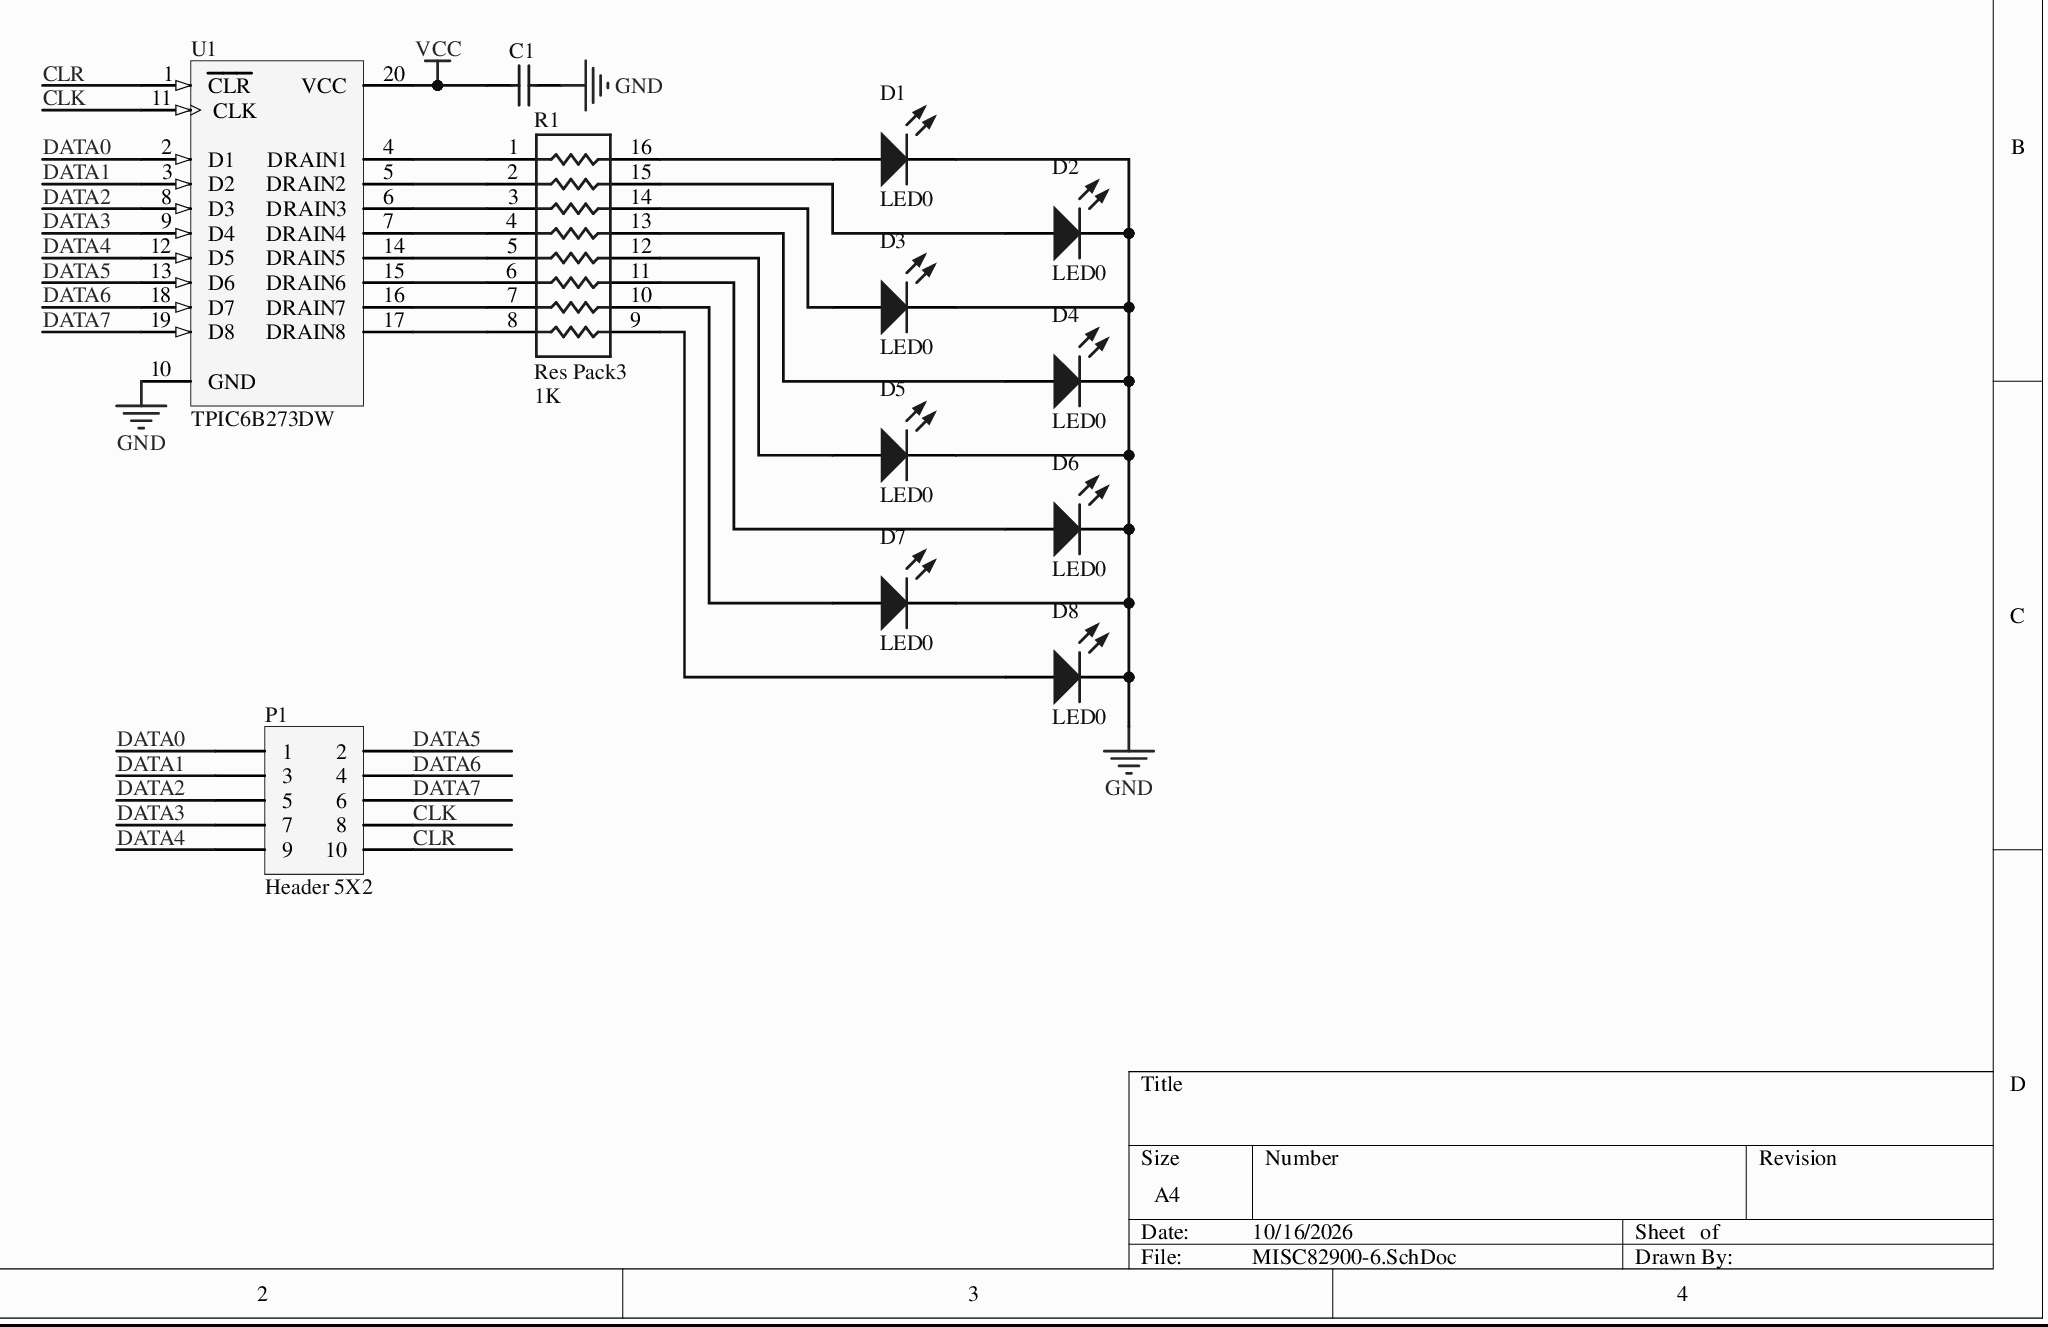
[diagram p0: MISC82900-6.SchDoc]
# Altium project MISC82900-2.PrjPcb
1 sheet, 12 parts. Net scope: global (net labels, ports and power ports of the same name join across sheets).
Board file: MISC82900.PcbDoc

## Sheet MISC82900-6.SchDoc
size A4

### Parts
C1  Cap  [RAD-0.3]  (value not drawn)
D1  LED0  [LED-0]
D2  LED0  [LED-0]
D3  LED0  [LED-0]
D4  LED0  [LED-0]
D5  LED0  [LED-0]
D6  LED0  [LED-0]
D7  LED0  [LED-0]
D8  LED0  [LED-0]
P1  Header 5X2  [HDR2X5]
R1  Res Pack3  value 1K  [SO-16_N]
U1  TPIC6B273DW  [DW020]

### Nets
GND: C1.2 D1.2(K) D2.2(K) D3.2(K) D4.2(K) D5.2(K) D6.2(K) D7.2(K) D8.2(K) U1.10(GND)
VCC: C1.1 U1.20(VCC)
CLK: P1.8 U1.11(CLK)
CLR: P1.10 U1.1(~{CLR})
DATA0: P1.1 U1.2(D1)
DATA1: P1.3 U1.3(D2)
DATA2: P1.5 U1.8(D3)
DATA3: P1.7 U1.9(D4)
DATA4: P1.9 U1.12(D5)
DATA5: P1.2 U1.13(D6)
DATA6: P1.4 U1.18(D7)
DATA7: P1.6 U1.19(D8)
NetD1_1: D1.1(A) R1.16
NetD2_1: D2.1(A) R1.15
NetD3_1: D3.1(A) R1.14
NetD4_1: D4.1(A) R1.13
NetD5_1: D5.1(A) R1.12
NetD6_1: D6.1(A) R1.11
NetD7_1: D7.1(A) R1.10
NetD8_1: D8.1(A) R1.9
NetR1_1: R1.1 U1.4(DRAIN1)
NetR1_2: R1.2 U1.5(DRAIN2)
NetR1_3: R1.3 U1.6(DRAIN3)
NetR1_4: R1.4 U1.7(DRAIN4)
NetR1_5: R1.5 U1.14(DRAIN5)
NetR1_6: R1.6 U1.15(DRAIN6)
NetR1_7: R1.7 U1.16(DRAIN7)
NetR1_8: R1.8 U1.17(DRAIN8)

### Library data of the parts
C1 = Cap: Capacitor; Value: 100pF; Published: 8-Jun-2000; LatestRevisionDate: 17-Jul-2002; LatestRevisionNote: Re-released for DXP Platform.; PackageReference: RAD-0.3; PackageDescription: Radial Cap, Thru-Hole; 2 Leads; 0.3 in Pin Spacing; Publisher: Altium Limited
D1-D8 = LED0: Typical INFRARED GaAs LED; Published: 8-Jun-2000; LatestRevisionDate: 08-Jul-2005; LatestRevisionNote: Mech Layer 1 removed.; PackageReference: LED-0; PackageDescription: LED; 2 Leads; Publisher: Altium Limited
P1 = Header 5X2: Header, 5-Pin, Dual row; LatestRevisionDate: 17-Jul-2002; LatestRevisionNote: Re-released for DXP Platform.; Publisher: Altium Limited
R1 = Res Pack3: Isolated Resistor Network; Published: 24-Mar-1999; LatestRevisionDate: 29-May-2009; LatestRevisionNote: IPC-7351 Footprint Added.; PackageReference: SO-16; PackageDescription: 16-Pin Small Outline Integrated Circuit 1.27 mm Pitch; Code_JEDEC: MS-012-AC; Code_IPC: SOIC127P600-16; Publisher: Altium Limited
U1 = TPIC6B273DW: Power Logic Octal D-Type Latch; Package Information: Latest Revision: Mar-2000; Code - JEDEC: MS-013; Published: 8-Jun-2000; Revision: 17-Jul-2002: Re-released for DXP Platform.; Datasheet: Latest Revision: Jul-1995; Package Reference: DW020; Publisher: Altium Limited